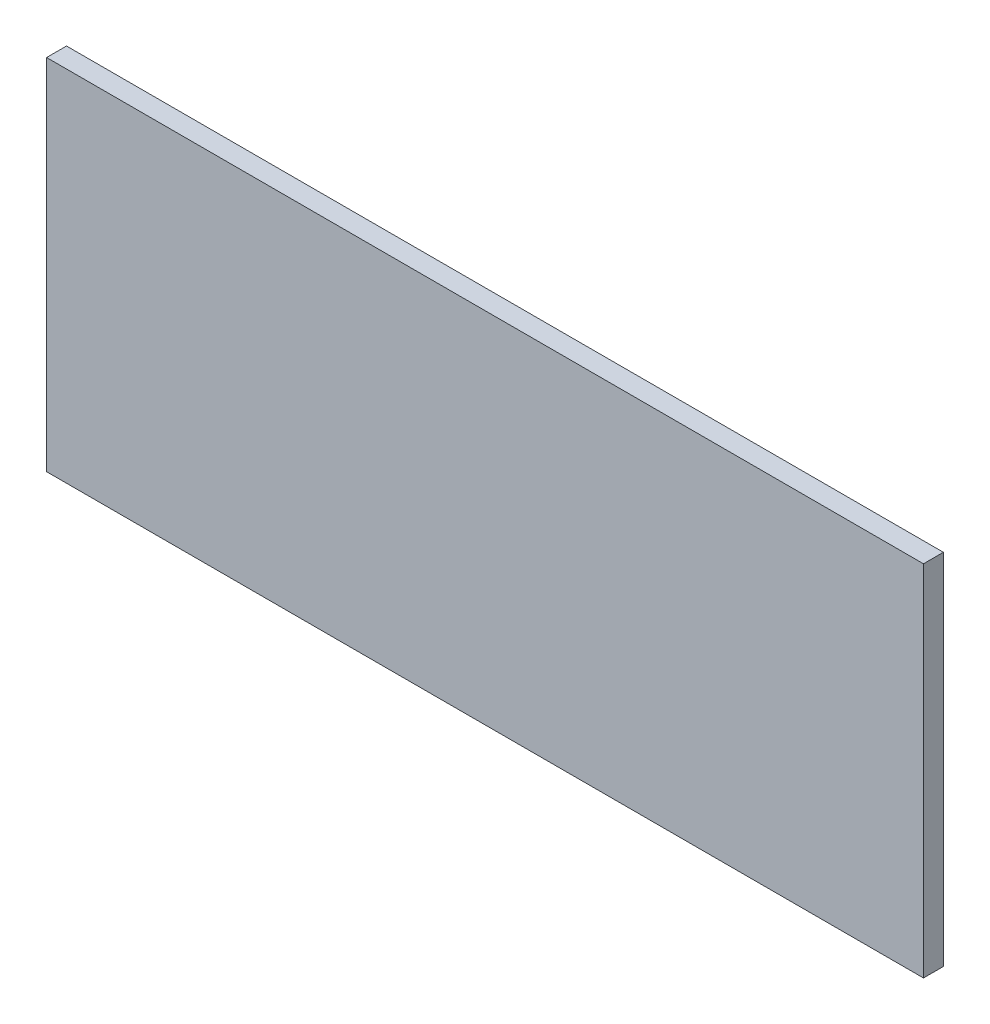
from build123d import *

# Parameters (mm, degrees)
SKETCH_1_W      = 440
SKETCH_1_H      = 180
EXTRUDE_1_DEPTH = 10


with BuildPart() as part:
    # 草图1 → 凸台-拉伸1 (new body)
    with BuildSketch(Plane.XY):
        with Locations((220, -90)):
            Rectangle(SKETCH_1_W, SKETCH_1_H)
    extrude(amount=EXTRUDE_1_DEPTH)


solid = part.part
